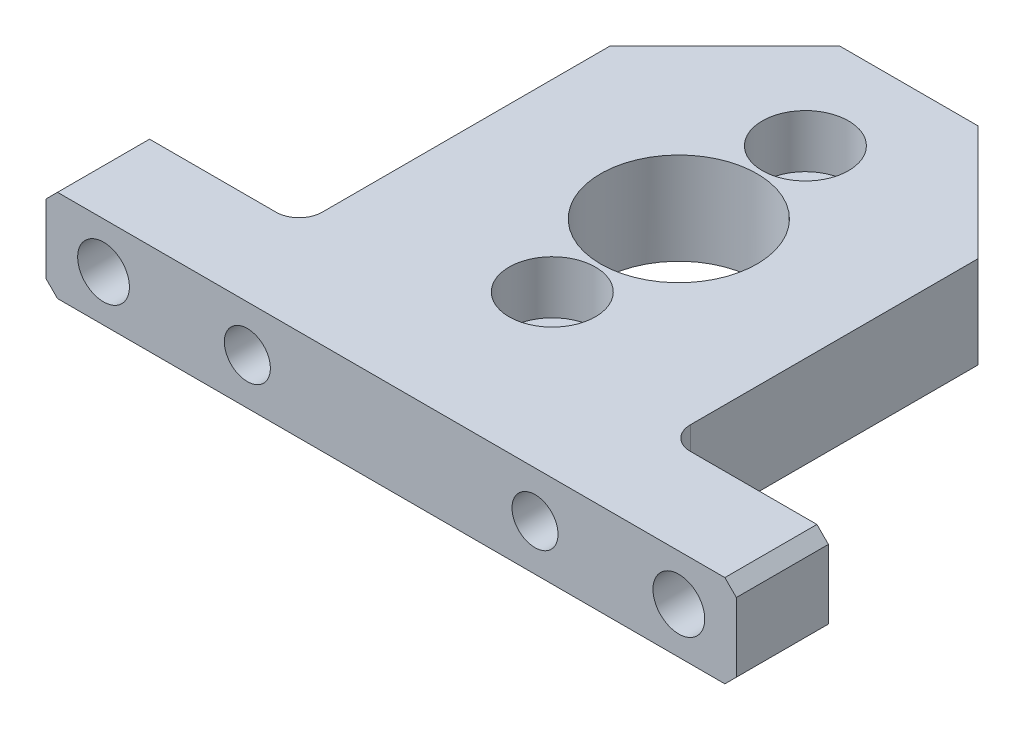
SolidWorks part; units mm, degrees
material "S45C"
ref_plane "前视基准面" through (0, 0, 0) normal (0, 0, 1) x (1, 0, 0)
ref_plane "上视基准面" through (0, 0, 0) normal (0, 1, 0) x (1, 0, 0)
ref_plane "右视基准面" through (0, 0, 0) normal (1, 0, 0) x (0, 0, -1)
sketch "草图1" plane through (0, 0, 0) normal (0, 1, 0) x (1, 0, 0)
  line L0 (-30, 0) -> (30, 0)
  line L1 (30, 0) -> (30, 8)
  line L2 (30, 8) -> (18, 8)
  line L3 (16, 10) -> (16, 45)
  line L4 (16, 45) -> (-16, 45)
  line L5 (-16, 45) -> (-16, 10)
  line L6 (-18, 8) -> (-30, 8)
  line L7 (-30, 8) -> (-30, 0)
  line L8 (0, 0) -> (0, 183.4286) construction
  arc A0 (-16, 10) -> (-18, 8) centre (-18, 10) cw
  arc A1 (18, 8) -> (16, 10) centre (18, 10) cw
  dimension "D5" = 2
  dimension "D1" = 32
  dimension "D2" = 60
  dimension "D3" = 45
  dimension "D4" = 8
extrude "凸台-拉伸1" add sketch "草图1" along normal mid plane 8
chamfer "倒角1" distance 1 angle 45 4 edges at (30, -4, -4) (30, 4, -4) (-30, -4, -4) (-30, 4, -4)
chamfer "倒角2" distance 10 angle 45 2 edges at (16, 0, -45) (-16, 0, -45)
sketch "草图2" plane through (0, 4, 0) normal (0, 1, 0) x (1, 0, 0)
  line L0 (-29, 0) -> (29, 0) construction
  circle A0 centre (0, 25) radius 6.8
  dimension "D1" = 13.6
  dimension "D2" = 25
extrude "切除-拉伸1" cut sketch "草图2" against normal up to next
sketch "草图5" plane through (0, 4, 0) normal (0, 1, 0) x (1, 0, 0)
  line L0 (0, 36) -> (0, 14) construction
  line L3 (0, 25) -> (0, 43.9063) construction
  circle A0 centre (0, 25) radius 11 construction
  point P0 (0, 36)
  point P2 (0, 14)
  dimension "D2" = 22
  dimension "D1" = 0
hole_wizard "M4 六角圆柱头螺钉的柱形沉头孔2" positions "草图5" profile "草图6" counterbore size "M4" standard "GB" end condition up to next
sketch "草图6" plane through (0, 4, -36) normal (1, 0, 0) x (0, 0, 1)
  line L0 (0, 0) -> (0, 8)
  line L1 (0, 8) -> (2.25, 8)
  line L3 (2.25, 8) -> (2.25, 4.6)
  line L4 (2.25, 4.6) -> (3.75, 4.6)
  line L5 (3.75, 4.6) -> (3.75, 0)
  line L7 (3.75, 0) -> (0, 0)
  line L11 (0, -6.35) -> (0, 107.95) construction
  dimension "通孔孔直径" = 4.5
  dimension "通孔孔深度" = 8
  dimension "柱形沉头孔直径" = 7.5
  dimension "柱形沉头孔深度" = 4.6
sketch "草图7" plane through (0, 0, 0) normal (0, 0, 1) x (1, 0, 0)
  line L0 (0, 0) -> (0, 7.7356) construction
  point P0 (-12.5, 0)
  point P2 (12.5, 0)
  dimension "D1" = 25
hole_wizard "Ø4.0mm 暗销孔1" positions "草图7" profile "草图8" hole size "Ø4.0" standard "GB"
sketch "草图8" plane through (-12.5, 0, 0) normal (1, 0, 0) x (0, -1, 0)
  line L0 (0, 0) -> (0, 11.2017)
  line L1 (0, 11.2017) -> (2, 10)
  line L2 (2, 10) -> (2, 0)
  line L5 (2, 0) -> (0, 0)
  line L10 (0, 11.2017) -> (-2, 10) construction
  line L11 (0, -6.35) -> (0, 107.95) construction
  dimension "孔直径" = 4
  dimension "孔深度" = 10
  dimension "导头角度" = 118
sketch "草图9" plane through (0, 0, -8) normal (0, 0, -1) x (-1, 0, 0)
  line L0 (0, 0) -> (0, 7.8696) construction
  point P0 (-25, 0)
  point P2 (25, 0)
  dimension "D1" = 50
hole_wizard "M4 间隙孔1" positions "草图9" profile "草图10" hole size "M4" standard "GB" end condition up to next
sketch "草图10" plane through (25, 0, -8) normal (1, 0, 0) x (0, 1, 0)
  line L0 (0, 0) -> (0, 8)
  line L1 (0, 8) -> (2.25, 8)
  line L2 (2.25, 8) -> (2.25, 0)
  line L5 (2.25, 0) -> (0, 0)
  line L11 (0, -6.35) -> (0, 107.95) construction
  dimension "通孔孔直径" = 4.5
  dimension "通孔孔深度" = 8
